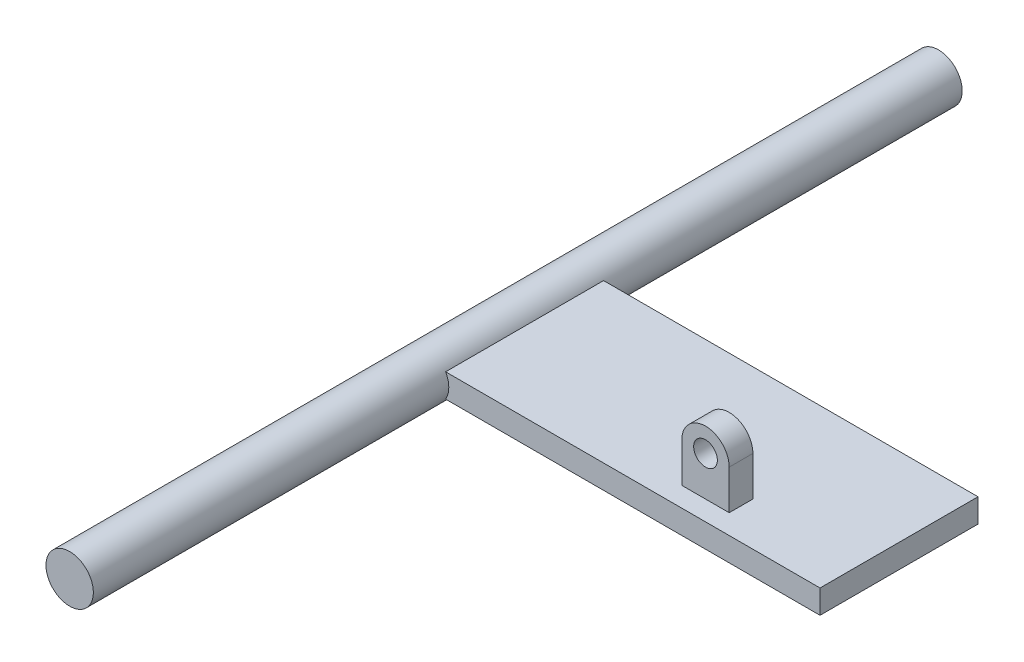
from build123d import *

# Parameters (mm, degrees)
SKETCH1_R           = 3
BOSS_EXTRUDE1_DEPTH = 55
SKETCH2_W           = 50
SKETCH2_H           = 3
BOSS_EXTRUDE2_DEPTH = 10
SKETCH3_R           = 3
SKETCH3_R_2         = 1.5
BOSS_EXTRUDE3_DEPTH = 3


with BuildPart() as part:
    # Sketch1 → Boss-Extrude1 (new, symmetric)
    with BuildSketch(Plane.XY):
        Circle(SKETCH1_R)
    extrude(amount=BOSS_EXTRUDE1_DEPTH, both=True)

    # Sketch2 → Boss-Extrude2 (add, symmetric)
    with BuildSketch(Plane.XY):
        with Locations((25, 0)):
            Rectangle(SKETCH2_W, SKETCH2_H)
    extrude(amount=BOSS_EXTRUDE2_DEPTH, both=True)

    # Sketch3 → Boss-Extrude3 (add)
    # profile 1 of 2: a face of its own
    with BuildSketch(Plane.XY.offset(7.5)):
        with Locations((33, 6.5)):
            Circle(SKETCH3_R)
        with Locations((33, 6.5)):
            Circle(SKETCH3_R_2, mode=Mode.SUBTRACT)
    # profile 2 of 2: a face of its own
    with BuildSketch(Plane.XY.offset(7.5)):
        with BuildLine():
            ThreePointArc((36, 6.5), (33, 3.5), (30, 6.5))
            Line((30, 6.5), (30, 1.5))
            Line((30, 1.5), (36, 1.5))
            Line((36, 1.5), (36, 6.5))
        make_face()
    extrude(amount=-BOSS_EXTRUDE3_DEPTH)


solid = part.part
